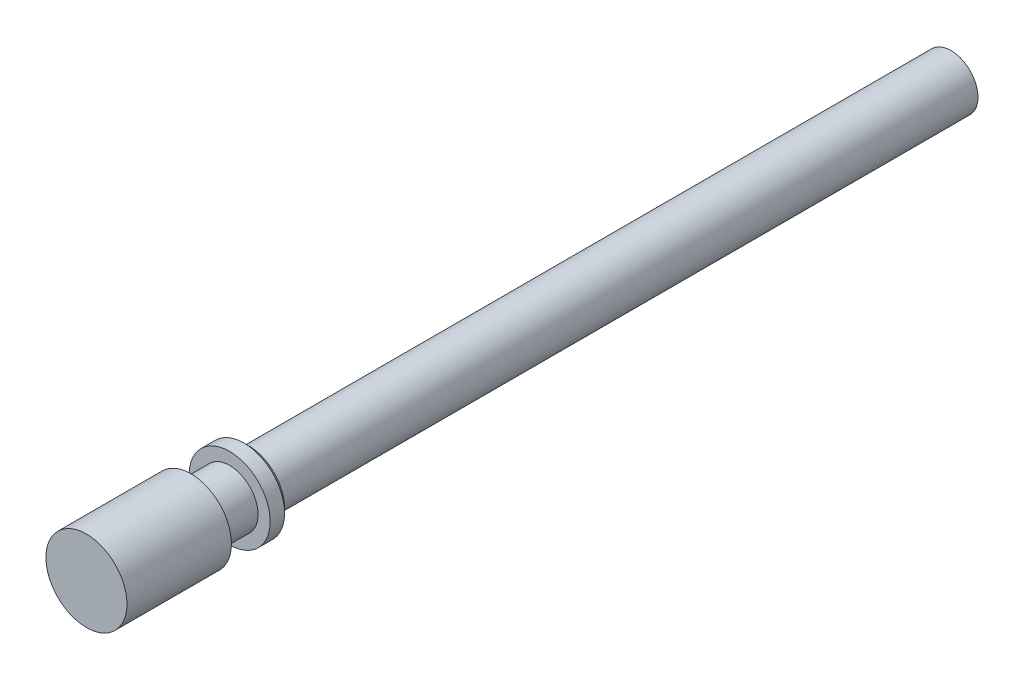
SolidWorks part; units mm, degrees
ref_plane "Front Plane" through (0, 0, 0) normal (0, 0, 1) x (1, 0, 0)
ref_plane "Top Plane" through (0, 0, 0) normal (0, 1, 0) x (1, 0, 0)
ref_plane "Right Plane" through (0, 0, 0) normal (1, 0, 0) x (0, 0, -1)
sketch "Sketch1" plane through (0, 0, 0) normal (0, 0, 1) x (1, 0, 0)
  circle A0 centre (0, 0) radius 3
  dimension "D1" = 6
extrude "Boss-Extrude1" add sketch "Sketch1" along normal blind 96
sketch "Sketch2" plane through (0, 0, 96) normal (0, 0, 1) x (1, 0, 0)
  circle A0 centre (0, 0) radius 4.5
  dimension "D1" = 9
extrude "Boss-Extrude2" add sketch "Sketch2" against normal blind 18
sketch "Sketch3" plane through (0, 0, 96) normal (0, 0, 1) x (1, 0, 0)
  circle A0 centre (0, 0) radius 3.15
  dimension "D1" = 6.3
extrude "Cut-Extrude1" cut sketch "Sketch3" against normal blind 4.3 from offset 11.6 flip side to cut offset against normal yes
chamfer "Chamfer1" distance 0.5 angle 45 1 edges at (4.5, 0, 78)
